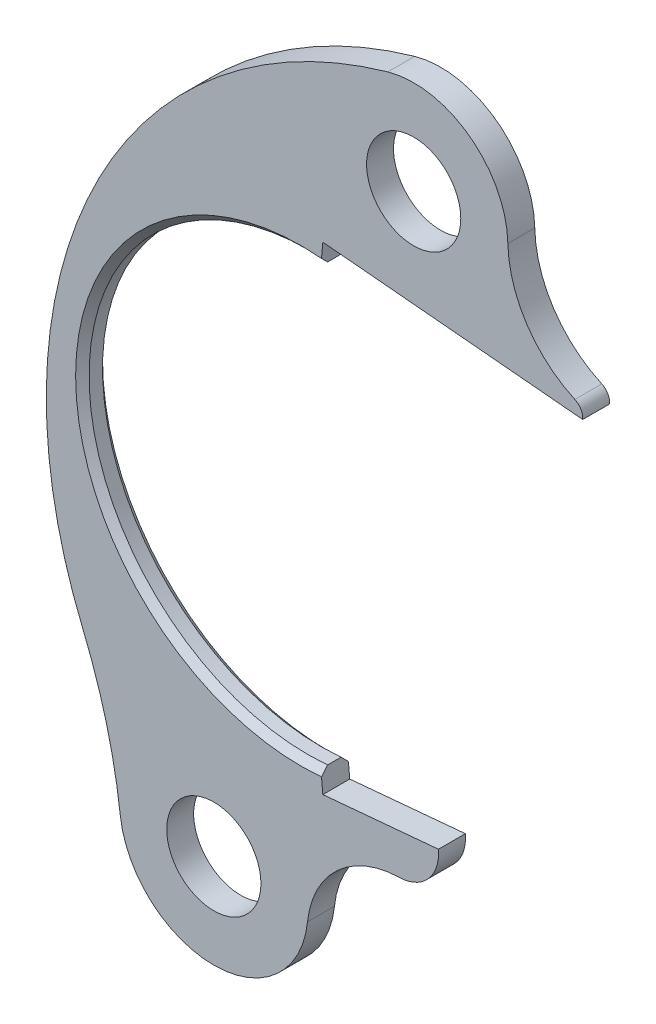
SolidWorks part; units mm, degrees
ref_plane "Front Plane" through (0, 0, 0) normal (0, 0, 1) x (1, 0, 0)
ref_plane "Top Plane" through (0, 0, 0) normal (0, 1, 0) x (1, 0, 0)
ref_plane "Right Plane" through (0, 0, 0) normal (1, 0, 0) x (0, 0, -1)
sketch "Sketch1" plane through (0, 0, 0) normal (0, 0, 1) x (1, 0, 0)
  line L0 (0, -294.832) -> (0, 341.6689) construction
  line L1 (-258.761, 0) -> (242.033, 0) construction
  line L2 (65.4941, 244.2) -> (442.5908, 244.2) construction
  line L3 (83.7, 429.3378) -> (83.7, 125.4988) construction
  line L4 (-95.4325, -258) -> (279.2623, -258) construction
  line L5 (-64.8, -221.5744) -> (-64.8, -378.8981) construction
  line L6 (16.2, 177.8) -> (209.3, 160.2)
  line L7 (16.2, 177.8) -> (14.7449, 161.8297)
  line L8 (16.2, -177.7) -> (102.1, -169.9)
  line L9 (16.2, -177.7) -> (14.7531, -161.8289)
  arc A0 (14.7449, 161.8297) -> (14.7531, -161.8289) centre (0, 0) ccw
  circle A1 centre (83.7, 244.2) radius 35
  arc A2 (153.6833, 245.73) -> (64.4462, 311.5) centre (83.7, 244.2) ccw
  circle A3 centre (-64.8, -258) radius 35
  arc A4 (-134.3064, -266.2983) -> (4.8189, -265.2942) centre (-64.8, -258) ccw
  arc A5 (-134.3064, -266.2983) -> (-162.3118, -159.7347) centre (-531.4857, -313.7173) ccw
  arc A6 (-64.8, -292.6618) -> (-64.4007, -292.9977) centre (160.7153, -25) ccw
  arc A7 (64.4462, 311.5) -> (-162.3118, -159.7347) centre (160.7153, -25) ccw
  arc A8 (209.3, 160.2) -> (203.4804, 170.2108) centre (199.3413, 161.1077) ccw
  arc A9 (153.6833, 245.73) -> (203.4804, 170.2108) centre (238.663, 247.5878) ccw
  arc A10 (72.8874, -202.6056) -> (102.1, -169.9) centre (72.2229, -172.6129) ccw
  arc A11 (72.8874, -202.6056) -> (4.8189, -265.2942) centre (74.4378, -272.5884) ccw
  dimension "D1" = 325
  dimension "D6" = 70
  dimension "D7" = 140
  dimension "D8" = 70
  dimension "D9" = 140
  dimension "D10" = 25
  dimension "D12" = 700
  dimension "D11" = 800
  dimension "D16" = 20
  dimension "D17" = 170
  dimension "D22" = 60
  dimension "D23" = 140
  dimension "D2" = 258
  dimension "D3" = 244.2
  dimension "D4" = 83.7
  dimension "D5" = 64.8
  dimension "D13" = 17.6
  dimension "D14" = 160.2
  dimension "D15" = 209.3
  dimension "D18" = 169.9
  dimension "D19" = 102.1
  dimension "D20" = 16.2
  dimension "D21" = 7.8
  dimension "D24" = 16.2
extrude "Boss-Extrude1" add sketch "Sketch1" along normal blind 20 contours A11 A10 L8 L9 A0 L7 L6 A8 A9 A2 A7 A5 A4 A3 A1
chamfer "Chamfer1" distance 5 angle 45 2 edges at (-162.5, -0.0041, 0) (-162.5, -0.0041, 20)
